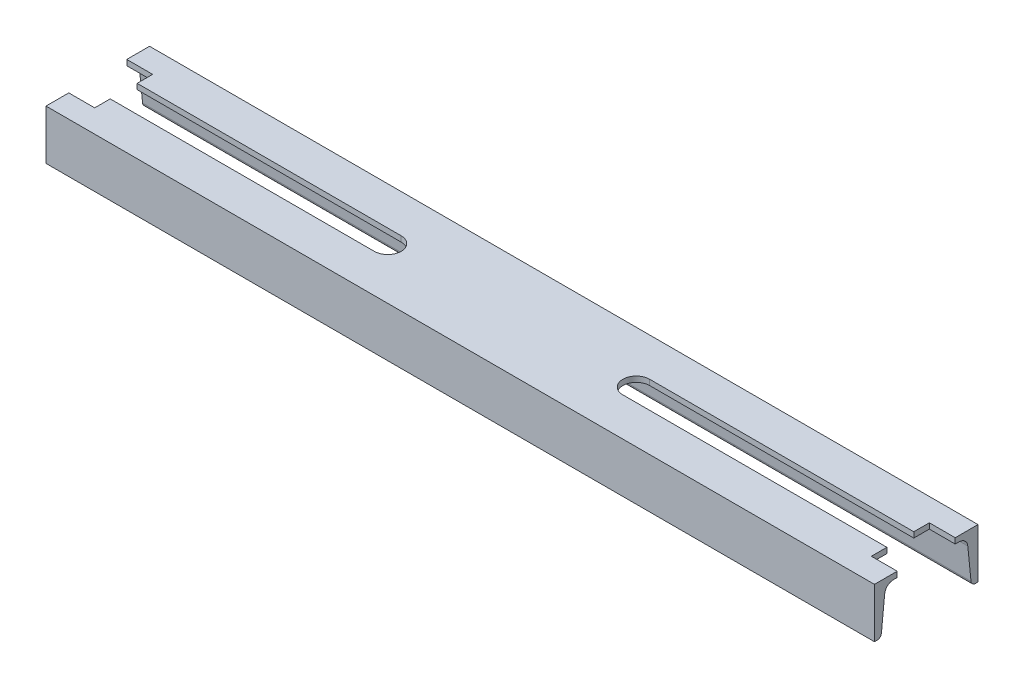
SolidWorks part; units mm, degrees
material "Q235-A"
ref_plane "Front Plane" through (0, 0, 0) normal (0, 0, 1) x (1, 0, 0)
ref_plane "Top Plane" through (0, 0, 0) normal (0, 1, 0) x (1, 0, 0)
ref_plane "Right Plane" through (0, 0, 0) normal (1, 0, 0) x (0, 0, -1)
sketch "草图1" plane through (0, 0, 0) normal (0, 0, 1) x (1, 0, 0)
  line L0 (400, 0) -> (-400, 0)
  point P4 (0, 0)
  dimension "D1" = 800
other "hot-rolled channel steel (GB/T 707-1988) 10(1)"
ref_plane "Plane1" through (400, 0, 0) normal (-1, 0, 0) x (0, -1, 0)
sketch "Sketch1" plane through (400, 0, 0) normal (-1, 0, 0) x (0, -1, 0)
  line L0 (48, 100) -> (0, 100)
  line L1 (48, 0) -> (0, 0)
  line L2 (0, 100) -> (0, 0)
  line L3 (54.084, 120.3761) -> (64.084, 120.3761) construction
  line L4 (54.084, 120.3761) -> (54.084, 119.3761) construction
  line L5 (54.084, 119.3761) -> (64.084, 120.3761) construction
  line L6 (48, 100) -> (48, 97.4812)
  line L7 (48, 0) -> (48, 2.5188)
  line L8 (0, 50) -> (5.3, 50) construction
  line L9 (26.65, 91.5) -> (26.65, 100) construction
  line L10 (5.3, 81.6726) -> (5.3, 91.5) construction
  line L11 (5.3, 91.5) -> (48, 91.5) construction
  line L12 (5.3, 81.6726) -> (5.3, 18.3274)
  line L13 (48, 91.5) -> (48, 100) construction
  line L17 (12.9542, 90.1304) -> (44.1729, 93.2523)
  line L18 (12.9542, 9.8696) -> (44.1729, 6.7477)
  arc A0 (44.1729, 93.2523) -> (48, 97.4812) centre (43.75, 97.4812) ccw
  arc A1 (44.1729, 6.7477) -> (48, 2.5188) centre (43.75, 2.5188) cw
  arc A9 (5.3, 18.3274) -> (12.9542, 9.8696) centre (13.8, 18.3274) ccw
  arc A10 (5.3, 81.6726) -> (12.9542, 90.1304) centre (13.8, 81.6726) cw
  point P8 (0, 50)
  point P9 (5.3, 50)
  point P10 (24, 100)
  point P11 (24, 0)
  point P12 (48, 6.365)
  point P13 (48, 93.635)
  point P27 (0, 0)
  dimension "D4" = 48
  dimension "D5" = 5.3
  dimension "D2" = 10
  dimension "D8" = 8.5
  dimension "D3" = 100
  dimension "D6" = 8.5
  dimension "D7" = 4.25
  dimension "D1" = 1
sketch "Sketch3" plane through (0, 0, 0) normal (0, 1, 0) x (1, 0, 0)
  line L0 (-680, -50) -> (-120, -50) construction
  line L1 (-400, -100) -> (-400, 0) construction
  line L2 (-680, -37) -> (-120, -37)
  line L3 (-680, -63) -> (-120, -63)
  arc A0 (-680, -37) -> (-680, -63) centre (-680, -50) ccw
  arc A1 (-120, -63) -> (-120, -37) centre (-120, -50) ccw
  point P4 (-400, -50)
  dimension "D1" = 13
  dimension "D2" = 280
extrude "Cut-Extrude1" cut sketch "Sketch3" against normal blind 10
sketch "Sketch4" plane through (0, 0, 0) normal (0, 1, 0) x (1, 0, 0)
  line L0 (-400, -22) -> (-375, -22)
  line L1 (-400, -37) -> (-400, 0) construction
  line L2 (-375, -22) -> (-375, -37)
  line L3 (-120, -37) -> (-400, -37) construction
  line L4 (-375, -37) -> (-400, -37)
  line L5 (-400, -37) -> (-400, -22)
  line L6 (-107, -50) -> (-624.2883, -50) construction
  line L7 (-400, -63) -> (-400, -78)
  line L8 (-375, -63) -> (-400, -63)
  line L9 (-375, -78) -> (-375, -63)
  line L10 (-400, -78) -> (-375, -78)
  arc A0 (-120, -63) -> (-120, -37) centre (-120, -50) ccw construction
  dimension "D1" = 15
  dimension "D2" = 25
extrude "Cut-Extrude2" cut sketch "Sketch4" against normal blind 10
mirror "Mirror1" about plane through (0, 0, 0) normal (1, 0, 0) of "Cut-Extrude2", "Cut-Extrude1"
